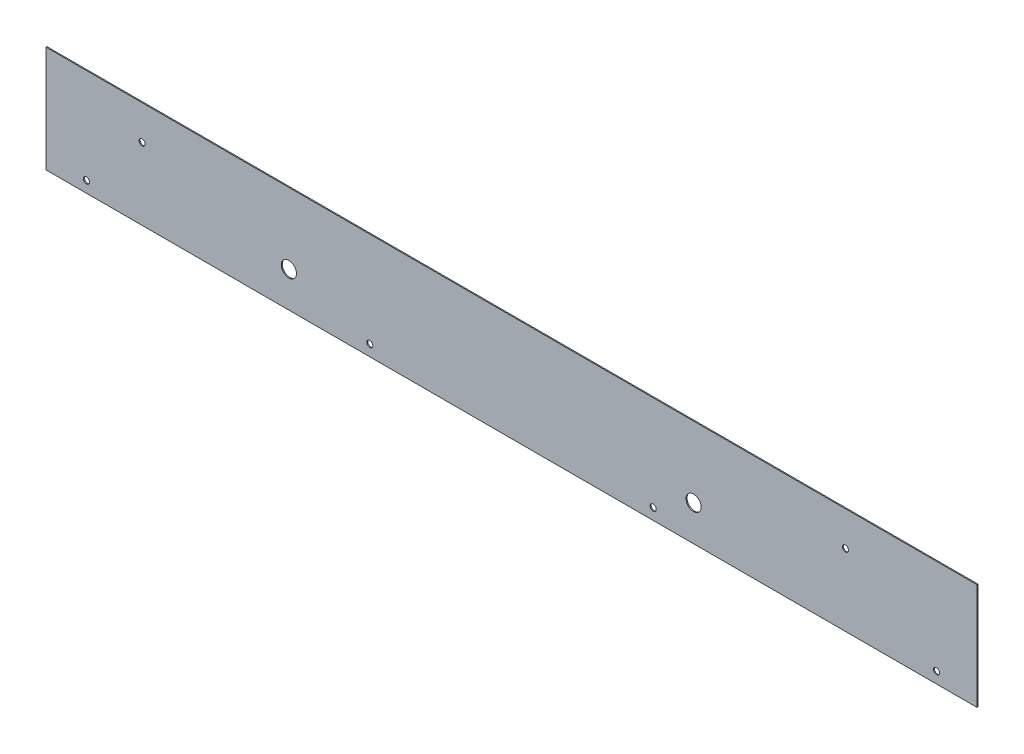
SolidWorks part; units mm, degrees
material "45#"
ref_plane "Front Plane" through (0, 0, 0) normal (0, 0, 1) x (1, 0, 0)
ref_plane "Top Plane" through (0, 0, 0) normal (0, 1, 0) x (1, 0, 0)
ref_plane "Right Plane" through (0, 0, 0) normal (1, 0, 0) x (0, 0, -1)
sketch "Sketch1" plane through (0, 0, 0) normal (0, 1, 0) x (1, 0, 0)
  line L0 (460, 0.5) -> (-460, -0.5) construction
  line L1 (-460, 0.5) -> (460, 0.5)
  line L2 (-460, 0.5) -> (-460, -0.5)
  line L3 (-460, -0.5) -> (460, -0.5)
  line L4 (460, 0.5) -> (460, -0.5)
  dimension "D1" = 920
  dimension "D2" = 1
extrude "Extrude1" add sketch "Sketch1" along normal mid plane 105
sketch "Sketch2" plane through (0, 0, 0.5) normal (0, 0, 1) x (1, 0, 0)
  line L0 (-460, -17.5) -> (-220, -17.5) construction
  line L1 (-460, 52.5) -> (-460, -52.5) construction
  line L2 (-220, -17.5) -> (180, -17.5) construction
  line L3 (-460, -52.5) -> (460, -52.5) construction
  circle A0 centre (-220, -17.5) radius 7.5
  circle A1 centre (180, -17.5) radius 7.5
  dimension "D3" = 15
  dimension "D1" = 240
  dimension "D2" = 400
  dimension "D4" = 35
extrude "Cut-Extrude1" cut sketch "Sketch2" against normal through all
hole_wizard "M5 Clearance Hole1" positions "Sketch5" profile "Sketch4" hole size "M5" standard "ISO"
sketch "Sketch5" plane through (0, 0, 0.5) normal (0, 0, 1) x (1, 0, 0)
  line L0 (-420, -41.5) -> (-140, -41.5) construction
  line L1 (-140, -41.5) -> (140, -41.5) construction
  line L3 (140, -41.5) -> (420, -41.5) construction
  line L5 (0, 0) -> (0, -41.5) construction
  line L7 (-460, -52.5) -> (460, -52.5) construction
  point P0 (-420, -41.5)
  point P1 (-140, -41.5)
  point P3 (140, -41.5)
  point P28 (-365, 18.5)
  point P31 (330, 18.5)
  point P36 (420, -41.5)
  point P41 (420, -41.5)
  dimension "D1" = 11
  dimension "D2" = 280
sketch "Sketch4" plane through (-420, -41.5, 0.5) normal (1, 0, 0) x (0, -1, 0)
  line L0 (0, 0) -> (0, 8.8026)
  line L1 (0, 8.8026) -> (3, 7)
  line L2 (3, 7) -> (3, 0)
  line L5 (3, 0) -> (0, 0)
  line L10 (0, 8.8026) -> (-3, 7) construction
  line L11 (0, -6.35) -> (0, 107.95) construction
  dimension "鑽孔直徑" = 6
  dimension "鑽孔深度" = 7
  dimension "導頭角度" = 118
